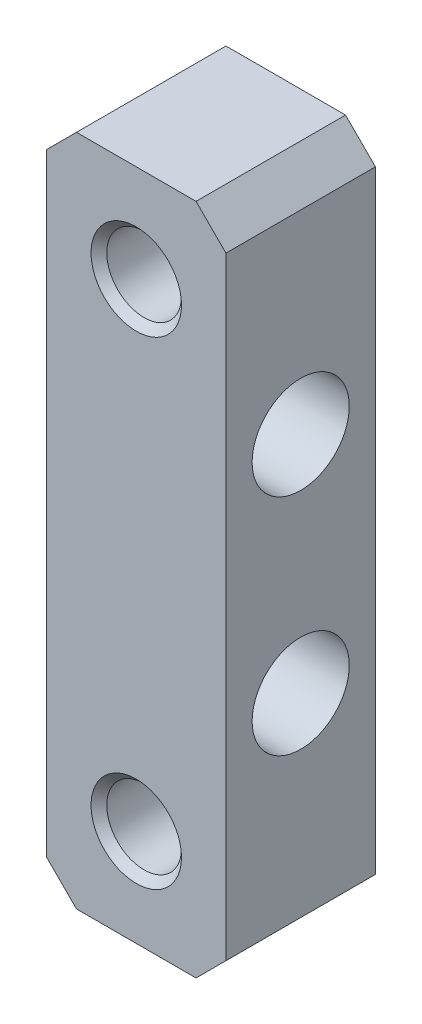
SolidWorks part; units mm, degrees
ref_plane "前视基准面" through (0, 0, 0) normal (0, 0, 1) x (1, 0, 0)
ref_plane "上视基准面" through (0, 0, 0) normal (0, 1, 0) x (1, 0, 0)
ref_plane "右视基准面" through (0, 0, 0) normal (1, 0, 0) x (0, 0, -1)
sketch "草图1" plane through (0, 0, 0) normal (0, 0, 1) x (1, 0, 0)
  line L1 (-6, -22.5) -> (6, -22.5)
  line L2 (-6, -22.5) -> (-6, 22.5)
  line L3 (-6, 22.5) -> (6, 22.5)
  line L4 (6, -22.5) -> (6, 22.5)
  line L5 (-6, -22.5) -> (6, 22.5) construction
  line L6 (-6, 22.5) -> (6, -22.5) construction
  point P0 (0, 0)
  dimension "D1" = 12
  dimension "D2" = 45
extrude "凸台-拉伸1" add sketch "草图1" along normal mid plane 10
hole_wizard "M6 螺纹孔1" positions "3D草图2" profile "草图2" tap size "M6" standard "GB" end condition up to next
sketch3d "3D草图2"
  line L0 (-6, -16, 5) -> (6, -16, 5)
  line L3 (6, -22.5, 5) -> (6, 22.5, 5) construction
  line L4 (-6, 22.5, 5) -> (-6, -22.5, 5) construction
  line L5 (-6, -22.5, 5) -> (6, -22.5, 5) construction
  point P0 (0, -16, 5)
  dimension "D1" = 6.5
sketch "草图2" plane through (0, -16, 5) normal (1, 0, 0) x (0, -1, 0)
  line L0 (0, 0) -> (0, 10.001)
  line L1 (0, 10.001) -> (2.5, 10.001)
  line L2 (2.5, 10.001) -> (2.5, 0.525)
  line L3 (2.5, 0.525) -> (3.025, 0)
  line L5 (3.025, 0) -> (0, 0)
  line L6 (-2.5, 0.525) -> (-3.025, 0) construction
  line L11 (0, -6.35) -> (0, 107.95) construction
  dimension "通孔螺纹孔钻头直径" = 5
  dimension "通孔螺纹孔钻头深度" = 10.001
  dimension "近端锥形沉头孔直径" = 6.05
  dimension "近端锥形沉头孔角度" = 90
cosmetic thread "孔螺蚊线1"
sketch "草图3" plane through (-6, 0, 0) normal (-1, 0, 0) x (0, 0, 1)
  line L0 (5, 22.5) -> (-5, 22.5) construction
  line L1 (5, -22.5) -> (-5, -22.5) construction
  circle A0 centre (0, 7.5) radius 3.25
  circle A1 centre (0, -7.5) radius 3.25
  dimension "D1" = 6.5
  dimension "D2" = 15
  dimension "D3" = 15
extrude "切除-拉伸1" cut sketch "草图3" against normal up to next
mirror "镜向1" about plane through (0, 0, 0) normal (0, 1, 0) of "M6 螺纹孔1"
chamfer "倒角1" distance 2 angle 45 4 edges at (-6, 22.5, 0) (6, 22.5, 0) (-6, -22.5, 0) (6, -22.5, 0)
